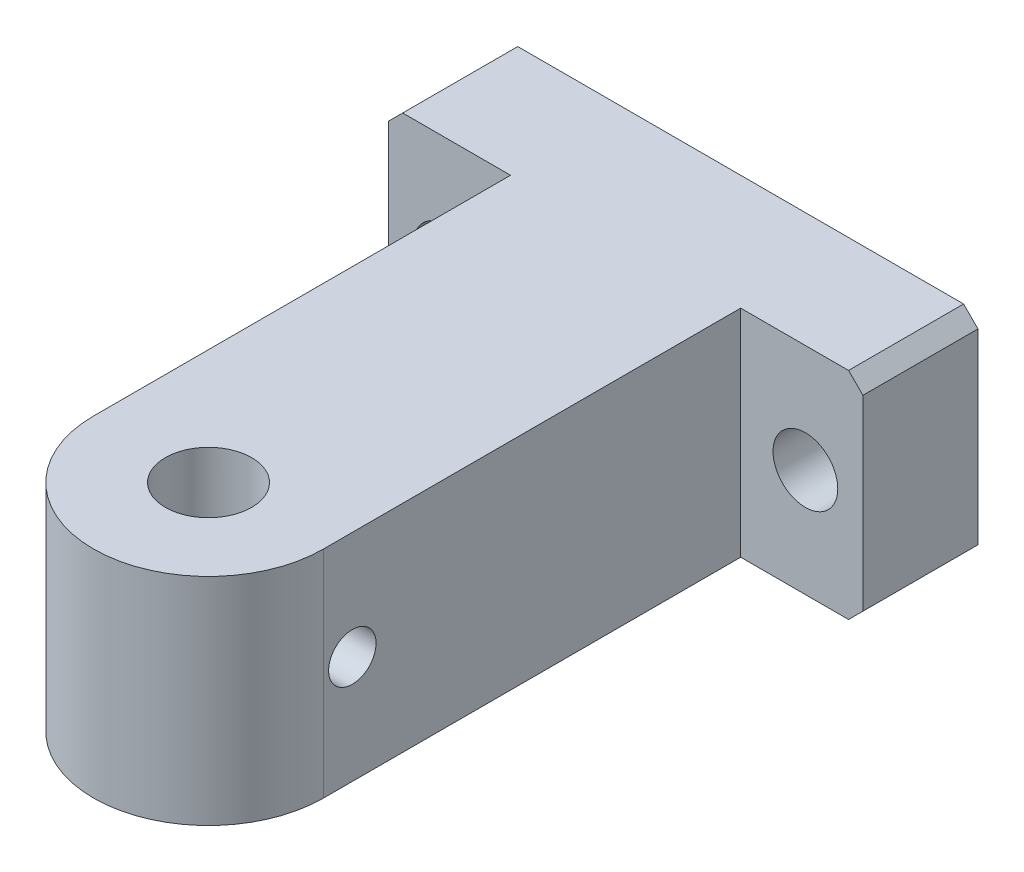
SolidWorks part; units mm, degrees
material "45钢"
ref_plane "前视基准面" through (0, 0, 0) normal (0, 0, 1) x (1, 0, 0)
ref_plane "上视基准面" through (0, 0, 0) normal (0, 1, 0) x (1, 0, 0)
ref_plane "右视基准面" through (0, 0, 0) normal (1, 0, 0) x (0, 0, -1)
sketch "草图1" plane through (0, 0, 0) normal (0, 1, 0) x (1, 0, 0)
  line L0 (0, 0) -> (0, 29) construction
  line L1 (-8, 0) -> (-8, 29)
  line L2 (8, 0) -> (8, 29)
  line L3 (8, 29) -> (16.5, 29)
  line L4 (16.5, 29) -> (16.5, 37)
  line L5 (16.5, 37) -> (-16.5, 37)
  line L6 (0, 20.0952) -> (0, 40.7239) construction
  line L7 (-16.5, 29) -> (-16.5, 37)
  line L8 (-8, 29) -> (-16.5, 29)
  circle A0 centre (0, 0) radius 3
  arc A1 (-8, 0) -> (8, 0) centre (0, 0) ccw
  point P3 (0, 12.9314)
  dimension "D1" = 6
  dimension "D2" = 8
  dimension "D3" = 37
  dimension "D4" = 16
  dimension "D5" = 33
extrude "凸台-拉伸1" add sketch "草图1" along normal mid plane 15
hole_wizard "M4 螺纹孔1" positions "草图2" profile "草图4" tap size "M4" standard "GB" end condition through all
sketch "草图2" plane through (8, 0, 0) normal (1, 0, 0) x (0, 0, -1)
  line L0 (37, 7.5) -> (37, -7.5) construction
  point P0 (2, 0)
  dimension "D1" = 35
sketch "草图4" plane through (8, 0, -2) normal (0, 1, 0) x (0, 0, -1)
  line L0 (0, 0) -> (0, 24.5)
  line L1 (0, 24.5) -> (1.65, 24.5)
  line L2 (1.65, 24.5) -> (1.65, 0)
  line L5 (1.65, 0) -> (0, 0)
  line L11 (0, -6.35) -> (0, 107.95) construction
  dimension "通孔螺纹孔钻头直径" = 3.3
  dimension "通孔螺纹孔钻头深度" = 24.5
cosmetic thread "孔螺蚊线1" parameters "D2"=4
sketch "草图5" plane through (0, 0, -29) normal (0, 0, 1) x (1, 0, 0)
  line L0 (-16.5, 7.5) -> (-16.5, -7.5) construction
  line L1 (0, -0.3535) -> (0, 9.2737) construction
  circle A0 centre (-12.5, 0) radius 2.25
  circle A1 centre (12.5, 0) radius 2.25
  dimension "D1" = 4
  dimension "D2" = 4.5
extrude "切除-拉伸1" cut sketch "草图5" against normal blind 10
chamfer "倒角1" distance 1 angle 45 4 edges at (-16.5, 7.5, -33) (-16.5, -7.5, -33) (16.5, -7.5, -33) (16.5, 7.5, -33)
